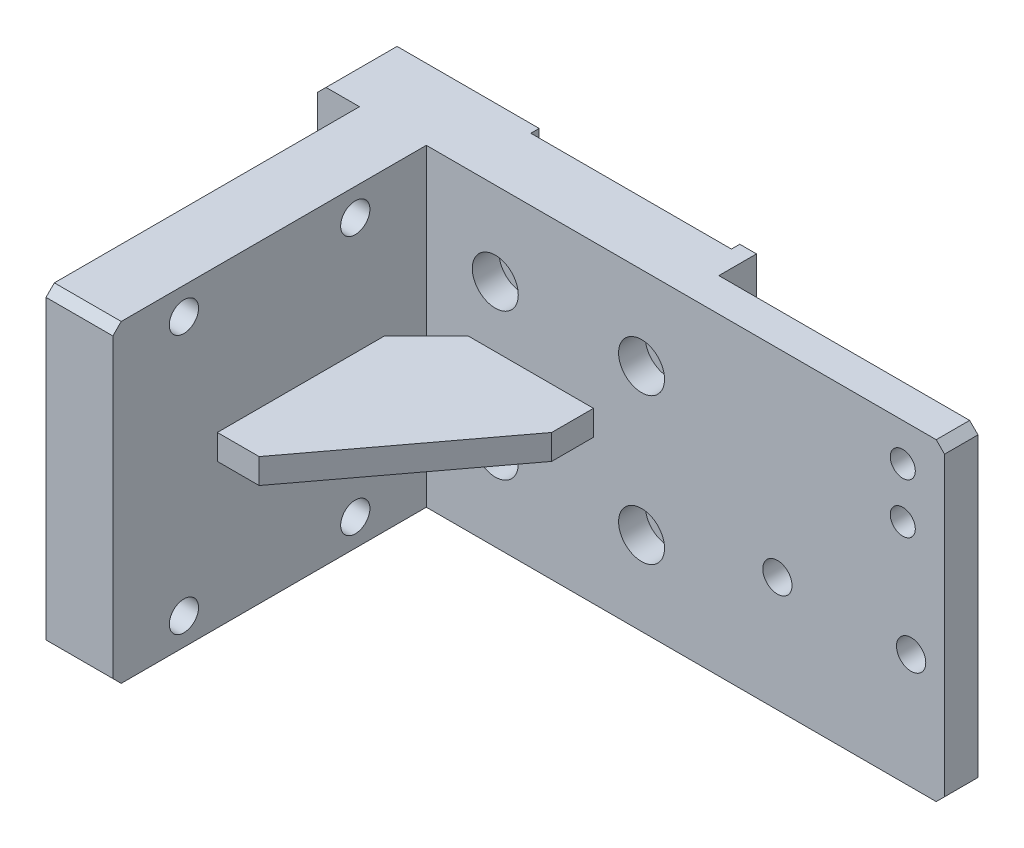
SolidWorks part; units mm, degrees
ref_plane "前视基准面" through (0, 0, 0) normal (0, 0, 1) x (1, 0, 0)
ref_plane "上视基准面" through (0, 0, 0) normal (0, 1, 0) x (1, 0, 0)
ref_plane "右视基准面" through (0, 0, 0) normal (1, 0, 0) x (0, 0, -1)
sketch "草图1" plane through (0, 0, 0) normal (0, 0, 1) x (1, 0, 0)
  line L1 (-75, 37.5) -> (75, 37.5)
  line L2 (-75, 37.5) -> (-75, -37.5)
  line L3 (-75, -37.5) -> (75, -37.5)
  line L4 (75, 37.5) -> (75, -37.5)
  line L5 (-75, 37.5) -> (75, -37.5) construction
  line L6 (-75, -37.5) -> (75, 37.5) construction
  point P0 (0, 0)
  dimension "D1" = 150
  dimension "D2" = 75
extrude "凸台-拉伸1" add sketch "草图1" along normal blind 17
hole_wizard "M6 六角凹头螺钉的柱形沉头孔1" positions "草图7" profile "草图6" counterbore size "M6" standard "ISO" end condition through all
sketch "草图7" plane through (0, 0, 17) normal (0, 0, 1) x (1, 0, 0)
  line L0 (-75, 37.5) -> (-75, -37.5) construction
  point P0 (2.5, 17.5)
  point P2 (-32.5, 17.5)
  point P4 (-32.5, -17.5)
  point P9 (2.5, -17.5)
  dimension "D1" = 42.5
  dimension "D2" = 35
  dimension "D3" = 35
  dimension "D4" = 17.5
sketch "草图6" plane through (2.5, 17.5, 17) normal (1, 0, 0) x (0, -1, 0)
  line L0 (0, 0) -> (0, 17)
  line L1 (0, 17) -> (3.3, 17)
  line L3 (3.3, 17) -> (3.3, 6.4)
  line L4 (3.3, 6.4) -> (5.5, 6.4)
  line L5 (5.5, 6.4) -> (5.5, 0)
  line L7 (5.5, 0) -> (0, 0)
  line L11 (0, -6.35) -> (0, 107.95) construction
  dimension "通孔孔直径" = 6.6
  dimension "通孔孔深度" = 17
  dimension "柱形沉头孔直径" = 11
  dimension "柱形沉头孔深度" = 6.4
sketch "草图8" plane through (0, 0, 17) normal (0, 0, 1) x (1, 0, 0)
  line L0 (75, 37.5) -> (-75, 37.5) construction
  line L1 (-65, 37.5) -> (-49, 37.5)
  line L2 (-65, 37.5) -> (-65, -37.5)
  line L3 (-65, -37.5) -> (-49, -37.5)
  line L4 (-49, 37.5) -> (-49, -37.5)
  line L5 (-75, -37.5) -> (75, -37.5) construction
  line L6 (-75, 37.5) -> (-75, -37.5) construction
  dimension "D1" = 16
  dimension "D2" = 10
extrude "凸台-拉伸2" add sketch "草图8" along normal blind 75
hole_wizard "Ø7.0 (7) 直径孔1" positions "草图10" profile "草图9" hole size "Ø7.0" standard "ISO" end condition through all
sketch "草图10" plane through (-49, 0, 0) normal (1, 0, 0) x (0, 0, -1)
  line L0 (0, -37.5) -> (0, 37.5) construction
  point P0 (-75, 31)
  point P2 (-75, -31)
  point P4 (-34, -31)
  point P6 (-34, 31)
  dimension "D1" = 34
  dimension "D2" = 41
  dimension "D3" = 62
  dimension "D4" = 31
sketch "草图9" plane through (-49, 31, 75) normal (0, 1, 0) x (0, 0, -1)
  line L0 (0, 0) -> (0, 26)
  line L1 (0, 26) -> (3.5, 26)
  line L2 (3.5, 26) -> (3.5, 0)
  line L5 (3.5, 0) -> (0, 0)
  line L11 (0, -6.35) -> (0, 107.95) construction
  dimension "通孔孔直径" = 7
  dimension "通孔孔深度" = 26
sketch "草图11" plane through (0, -37.5, 0) normal (0, -1, 0) x (1, 0, 0)
  line L0 (-75, 0) -> (75, 0) construction
  line L1 (-39, 0) -> (9, 0)
  line L2 (-39, 0) -> (-39, 2)
  line L3 (-39, 2) -> (9, 2)
  line L4 (9, 0) -> (9, 2)
  line L5 (-75, 17) -> (-75, 0) construction
  dimension "D1" = 48
  dimension "D2" = 2
  dimension "D3" = 36
extrude "切除-拉伸1" cut sketch "草图11" against normal through all
sketch "草图12" plane through (0, 0, 0) normal (0, 1, 0) x (1, 0, 0)
  line L0 (-49, -67) -> (-39, -67)
  line L1 (-49, -92) -> (-49, -17) construction
  line L2 (-39, -67) -> (-9, -27)
  line L3 (-9, -27) -> (-9, -17)
  line L4 (-49, -17) -> (75, -17) construction
  line L5 (-49, -27) -> (-39, -17)
  line L6 (-49, -67) -> (-49, -27)
  line L7 (-39, -17) -> (-9, -17)
  dimension "D1" = 10
  dimension "D2" = 10
  dimension "D3" = 30
  dimension "D4" = 10
  dimension "D5" = 10
  dimension "D6" = 50
extrude "凸台-拉伸3" add sketch "草图12" along normal mid plane 6
chamfer "倒角1" distance 2 angle 45 6 edges at (75, -37.5, 8.5) (75, 37.5, 8.5) (-57, -37.5, 92) (-57, 37.5, 92) (-75, 37.5, 8.5) (-75, -37.5, 8.5)
sketch "草图13" plane through (0, -37.5, 0) normal (0, -1, 0) x (1, 0, 0)
  line L1 (75, 0) -> (13, 0)
  line L2 (75, 0) -> (75, 9)
  line L3 (75, 9) -> (13, 9)
  line L4 (13, 0) -> (13, 9)
  dimension "D1" = 62
  dimension "D2" = 9
extrude "切除-拉伸2" cut sketch "草图13" against normal through all contours L3 L4 L1 L2
hole_wizard "Ø7.0 (7) 直径孔2" positions "草图15" profile "草图14" hole size "Ø7.0" standard "GB" end condition through all
sketch "草图15" plane through (0, 0, 17) normal (0, 0, 1) x (1, 0, 0)
  point P0 (35, -10)
  point P3 (67, -10)
sketch "草图14" plane through (35, -10, 17) normal (1, 0, 0) x (0, -1, 0)
  line L0 (0, 0) -> (0, 17)
  line L1 (0, 17) -> (3.5, 17)
  line L2 (3.5, 17) -> (3.5, 0)
  line L5 (3.5, 0) -> (0, 0)
  line L11 (0, -6.35) -> (0, 107.95) construction
  dimension "通孔孔直径" = 7
  dimension "通孔孔深度" = 17
hole_wizard "Ø6.0 (6) 直径孔1" positions "草图17" profile "草图16" hole size "Ø6.0" standard "GB" end condition through all
sketch "草图17" plane through (0, 0, 17) normal (0, 0, 1) x (1, 0, 0)
  point P0 (65, 28.5)
  point P3 (65, 16.5)
sketch "草图16" plane through (65, 28.5, 17) normal (1, 0, 0) x (0, -1, 0)
  line L0 (0, 0) -> (0, 17)
  line L1 (0, 17) -> (3, 17)
  line L2 (3, 17) -> (3, 0)
  line L5 (3, 0) -> (0, 0)
  line L11 (0, -6.35) -> (0, 107.95) construction
  dimension "通孔孔直径" = 6
  dimension "通孔孔深度" = 17
